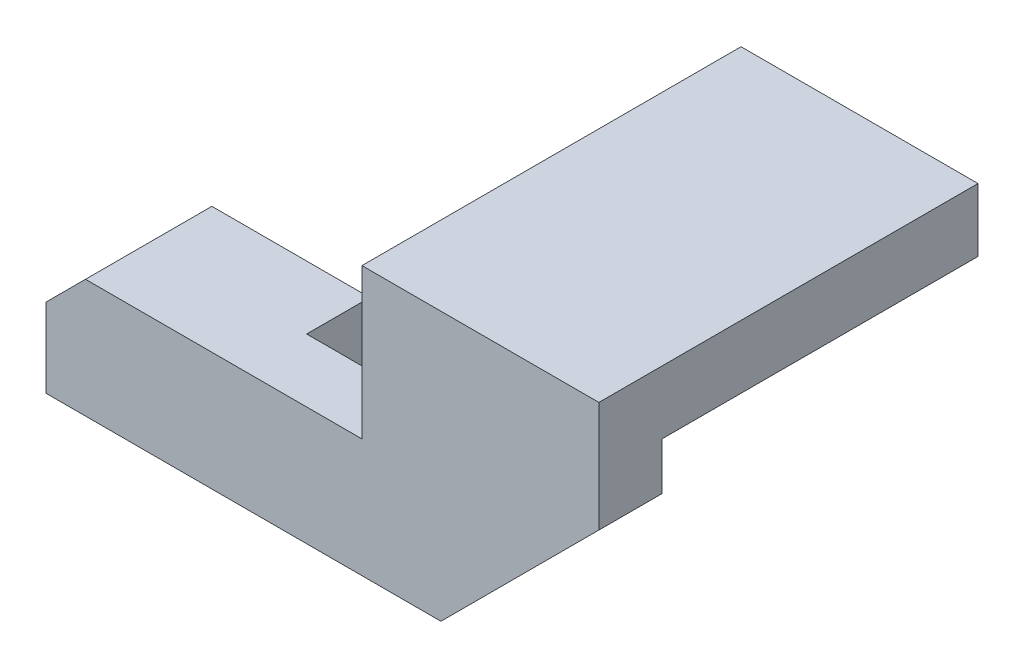
from build123d import *

# Parameters (mm, degrees)
SKETCH1_W           = 30
SKETCH1_H           = 40
BOSS_EXTRUDE1_DEPTH = 8
SKETCH2_W           = 30
SKETCH2_H           = 34
BOSS_EXTRUDE2_DEPTH = 8
SKETCH3_W           = 8
SKETCH3_H           = 15
BOSS_EXTRUDE3_DEPTH = 40
CHAMFER1_SIZE       = 5
BOSS_EXTRUDE4_DEPTH = 8
CHAMFER2_SIZE       = 20


with BuildPart() as part:
    # Sketch1 → Boss-Extrude1 (new body)
    with BuildSketch(Plane(origin=(0, 0, 0), x_dir=(1, 0, 0), z_dir=(0, 1, 0))):
        Rectangle(SKETCH1_W, SKETCH1_H)
    extrude(amount=BOSS_EXTRUDE1_DEPTH)

    # Sketch2 → Boss-Extrude2 (add)
    with BuildSketch(Plane.XY.offset(20)):
        with Locations((0, -9)):
            Rectangle(SKETCH2_W, SKETCH2_H)
    extrude(amount=BOSS_EXTRUDE2_DEPTH)

    # Sketch3 → Boss-Extrude3 (add)
    with BuildSketch(Plane.ZY.offset(15)):
        with Locations((24, -18.5)):
            Rectangle(SKETCH3_W, SKETCH3_H)
    extrude(amount=BOSS_EXTRUDE3_DEPTH)

    # Chamfer1
    chamfer1_edges = [part.edges().sort_by_distance(p)[0] for p in [
        (-55, -11, 24),
    ]]
    chamfer(chamfer1_edges, length=CHAMFER1_SIZE)

    # Sketch4 → Boss-Extrude4 (add)
    with BuildSketch(Plane(origin=(0, 0, 20), x_dir=(-1, 0, 0), z_dir=(0, 0, -1))):
        Polygon((30, -11), (50, -11), (55, -16), (55, -26), (30, -26), align=None)
    extrude(amount=BOSS_EXTRUDE4_DEPTH)

    # Chamfer2
    chamfer2_edges = [part.edges().sort_by_distance(p)[0] for p in [
        (15, -26, 24),
    ]]
    chamfer(chamfer2_edges, length=CHAMFER2_SIZE)


solid = part.part
